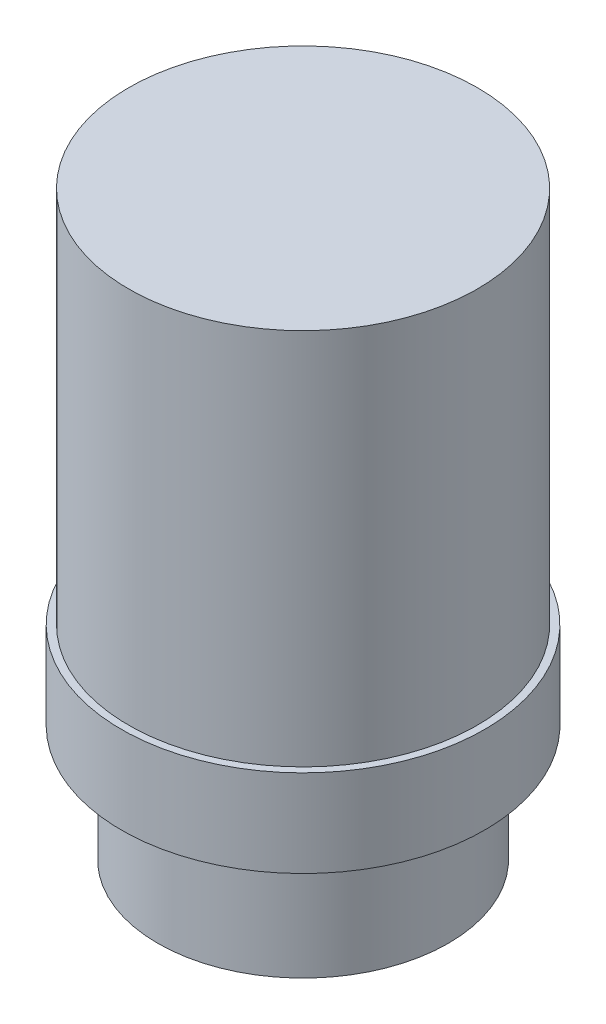
from build123d import *


with BuildPart() as part:
    # Sketch1 → Revolve1 (revolve)
    with BuildSketch(Plane.XY, mode=Mode.PRIVATE) as revolve1_sk:
        Polygon((0, 40), (-12, 40), (-12, 14), (-12.5, 14), (-12.5, 8), (-10, 8), (-10, 0), (0, 0), align=None)
    revolve(revolve1_sk.sketch.rotate(Axis((0, 0, 0), (0, 1, 0)), 270), axis=Axis((0, 0, 0), (0, 1, 0)))


solid = part.part
